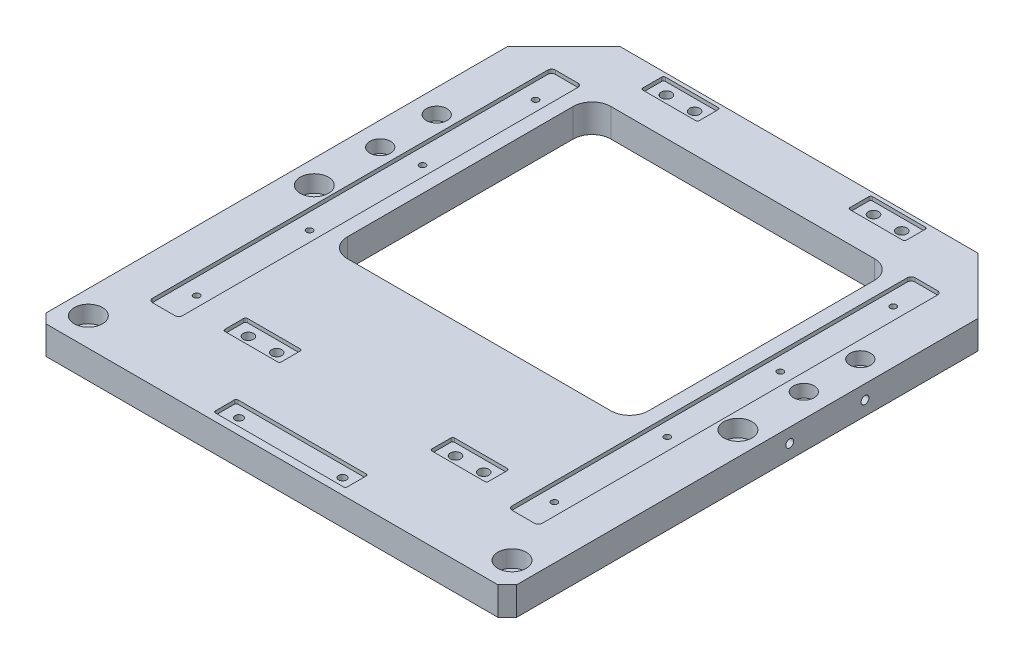
from build123d import *

# Parameters (mm, degrees)
SKETCH_1_W                   = 250
SKETCH_1_H                   = 280
EXTRUDE_1_DEPTH              = 7.5
HOLE_WIZARD_M8_2_D           = 9
HOLE_WIZARD_M8_2_CBORE_D     = 15
HOLE_WIZARD_M8_2_CBORE_DEPTH = 9
CUT_EXTRUDE_1_DEPTH          = 15
HOLE_WIZARD_M4_1_D           = 3.3
HOLE_WIZARD_M5_1_D           = 4.2
HOLE_WIZARD_M5_2_D           = 5.5
HOLE_WIZARD_M5_2_CBORE_D     = 10
HOLE_WIZARD_M5_2_CBORE_DEPTH = 5.7
CUT_EXTRUDE_2_DEPTH          = 2
HOLE_WIZARD_M6_1_D           = 6.6
HOLE_WIZARD_M6_1_DEPTH       = 15
HOLE_WIZARD_M6_1_CBORE_D     = 11
HOLE_WIZARD_M6_1_CBORE_DEPTH = 6.8
HOLE_WIZARD_M6_1_TIP         = 1.982840043
CUT_EXTRUDE_3_DEPTH          = 2
CUT_EXTRUDE_4_DEPTH          = 2
CHAMFER_1_SIZE               = 5
CHAMFER_2_SIZE               = 30
HOLE_WIZARD_M5_2_2_D         = 4.2
HOLE_WIZARD_M5_2_2_DEPTH     = 12.4
HOLE_WIZARD_M5_2_2_TIP       = 1.2618073


with BuildPart() as part:
    # 草图1 → 凸台-拉伸1 (new, symmetric)
    with BuildSketch(Plane(origin=(0, 0, 0), x_dir=(1, 0, 0), z_dir=(0, 1, 0))):
        Rectangle(SKETCH_1_W, SKETCH_1_H)
    extrude(amount=EXTRUDE_1_DEPTH, both=True)

    # M8 六角圆柱头螺钉的柱形沉头孔2 (through all)
    with Locations(Plane(origin=(0, 7.5, 0), x_dir=(1, 0, 0), z_dir=(0, 1, 0))):
        with Locations((-112.5, -125), (112.5, -125), (112.5, -5), (-112.5, -5)):
            CounterBoreHole(HOLE_WIZARD_M8_2_D / 2, HOLE_WIZARD_M8_2_CBORE_D / 2, HOLE_WIZARD_M8_2_CBORE_DEPTH)

    # 草图4 → 切除-拉伸1 (cut)
    with BuildSketch(Plane(origin=(0, 7.5, 0), x_dir=(1, 0, 0), z_dir=(0, 1, 0))):
        with BuildLine():
            Line((-70, -30), (70, -30))
            ThreePointArc((70, -30), (77.071067812, -27.071067812), (80, -20))
            Line((80, -20), (80, 100))
            ThreePointArc((80, 100), (77.071067812, 107.071067812), (70, 110))
            Line((70, 110), (-70, 110))
            ThreePointArc((-70, 110), (-77.071067812, 107.071067812), (-80, 100))
            Line((-80, 100), (-80, -20))
            ThreePointArc((-80, -20), (-77.071067812, -27.071067812), (-70, -30))
        make_face()
    extrude(amount=-CUT_EXTRUDE_1_DEPTH, mode=Mode.SUBTRACT)

    # M4 螺纹孔1 (through all)
    with Locations(Plane(origin=(0, 7.5, 0), x_dir=(1, 0, 0), z_dir=(0, 1, 0))):
        with Locations((95, 95), (-95, 95), (-95, 35), (-95, -25), (-95, -85), (95, 35), (95, -25), (95, -85)):
            Hole(HOLE_WIZARD_M4_1_D / 2)

    # M5 螺纹孔1 (through all)
    with Locations(Plane(origin=(0, 7.5, 0), x_dir=(1, 0, 0), z_dir=(0, 1, 0))):
        with Locations((27.5, -130), (-27.5, -130)):
            Hole(HOLE_WIZARD_M5_1_D / 2)

    # Hole Wizard M5 _2 (through all)
    with Locations(Plane(origin=(0, -7.5, 0), x_dir=(-1, 0, 0), z_dir=(0, -1, 0))):
        with Locations((47.5, 132), (62.5, 132), (62.5, -90), (47.5, -90), (-47.5, -90), (-62.5, -90), (-62.5, 132), (-47.5, 132)):
            CounterBoreHole(HOLE_WIZARD_M5_2_D / 2, HOLE_WIZARD_M5_2_CBORE_D / 2, HOLE_WIZARD_M5_2_CBORE_DEPTH)

    # 草图11 → 切除-拉伸2 (cut)
    with BuildSketch(Plane(origin=(0, 7.5, 0), x_dir=(1, 0, 0), z_dir=(0, 1, 0))):
        with BuildLine():
            Line((101.5, -102), (89.5, -102))
            ThreePointArc((89.5, -102), (88.085786438, -101.414213562), (87.5, -100))
            Line((87.5, -100), (87.5, 110))
            ThreePointArc((87.5, 110), (88.085786438, 111.414213562), (89.5, 112))
            Line((89.5, 112), (101.5, 112))
            ThreePointArc((101.5, 112), (102.914213562, 111.414213562), (103.5, 110))
            Line((103.5, 110), (103.5, -100))
            ThreePointArc((103.5, -100), (102.914213562, -101.414213562), (101.5, -102))
        make_face()
        with BuildLine():
            Line((-87.5, -100), (-87.5, 110))
            ThreePointArc((-87.5, 110), (-88.085786438, 111.414213562), (-89.5, 112))
            Line((-89.5, 112), (-101.5, 112))
            ThreePointArc((-101.5, 112), (-102.914213562, 111.414213562), (-103.5, 110))
            Line((-103.5, 110), (-103.5, -100))
            ThreePointArc((-103.5, -100), (-102.914213562, -101.414213562), (-101.5, -102))
            Line((-101.5, -102), (-89.5, -102))
            ThreePointArc((-89.5, -102), (-88.085786438, -101.414213562), (-87.5, -100))
        make_face()
    extrude(amount=-CUT_EXTRUDE_2_DEPTH, mode=Mode.SUBTRACT)

    # M6 六角圆柱头螺钉的柱形沉头孔1
    with Locations(Plane(origin=(0, 7.5, 0), x_dir=(1, 0, 0), z_dir=(0, 1, 0))):
        with Locations((-112.5, 30), (-112.5, 60), (112.5, 60), (112.5, 30)):
            CounterBoreHole(HOLE_WIZARD_M6_1_D / 2, HOLE_WIZARD_M6_1_CBORE_D / 2, HOLE_WIZARD_M6_1_CBORE_DEPTH, depth=HOLE_WIZARD_M6_1_DEPTH)
            with Locations((0, 0, -(HOLE_WIZARD_M6_1_DEPTH + HOLE_WIZARD_M6_1_TIP / 2))):  # 118° drill point
                Cone(0, HOLE_WIZARD_M6_1_D / 2, HOLE_WIZARD_M6_1_TIP, mode=Mode.SUBTRACT)

    # 草图14 → 切除-拉伸3 (cut)
    with BuildSketch(Plane(origin=(0, 7.5, 0), x_dir=(1, 0, 0), z_dir=(0, 1, 0))):
        with BuildLine():
            Line((-41, 138), (-69, 138))
            ThreePointArc((-69, 138), (-69.707106781, 137.707106781), (-70, 137))
            Line((-70, 137), (-70, 127))
            ThreePointArc((-70, 127), (-69.707106781, 126.292893219), (-69, 126))
            Line((-69, 126), (-41, 126))
            ThreePointArc((-41, 126), (-40.292893219, 126.292893219), (-40, 127))
            Line((-40, 127), (-40, 137))
            ThreePointArc((-40, 137), (-40.292893219, 137.707106781), (-41, 138))
        make_face()
        with BuildLine():
            Line((70, 137), (70, 127))
            ThreePointArc((70, 127), (69.707106781, 126.292893219), (69, 126))
            Line((69, 126), (41, 126))
            ThreePointArc((41, 126), (40.292893219, 126.292893219), (40, 127))
            Line((40, 127), (40, 137))
            ThreePointArc((40, 137), (40.292893219, 137.707106781), (41, 138))
            Line((41, 138), (69, 138))
            ThreePointArc((69, 138), (69.707106781, 137.707106781), (70, 137))
        make_face()
        with BuildLine():
            Line((41, -96), (69, -96))
            ThreePointArc((69, -96), (69.707106781, -95.707106781), (70, -95))
            Line((70, -95), (70, -85))
            ThreePointArc((70, -85), (69.707106781, -84.292893219), (69, -84))
            Line((69, -84), (41, -84))
            ThreePointArc((41, -84), (40.292893219, -84.292893219), (40, -85))
            Line((40, -85), (40, -95))
            ThreePointArc((40, -95), (40.292893219, -95.707106781), (41, -96))
        make_face()
        with BuildLine():
            Line((-70, -95), (-70, -85))
            ThreePointArc((-70, -85), (-69.707106781, -84.292893219), (-69, -84))
            Line((-69, -84), (-41, -84))
            ThreePointArc((-41, -84), (-40.292893219, -84.292893219), (-40, -85))
            Line((-40, -85), (-40, -95))
            ThreePointArc((-40, -95), (-40.292893219, -95.707106781), (-41, -96))
            Line((-41, -96), (-69, -96))
            ThreePointArc((-69, -96), (-69.707106781, -95.707106781), (-70, -95))
        make_face()
    extrude(amount=-CUT_EXTRUDE_3_DEPTH, mode=Mode.SUBTRACT)

    # 草图15 → 切除-拉伸4 (cut)
    with BuildSketch(Plane(origin=(0, 7.5, 0), x_dir=(1, 0, 0), z_dir=(0, 1, 0))):
        with BuildLine():
            Line((34, -124), (-34, -124))
            ThreePointArc((-34, -124), (-34.707106781, -124.292893219), (-35, -125))
            Line((-35, -125), (-35, -135))
            ThreePointArc((-35, -135), (-34.707106781, -135.707106781), (-34, -136))
            Line((-34, -136), (34, -136))
            ThreePointArc((34, -136), (34.707106781, -135.707106781), (35, -135))
            Line((35, -135), (35, -125))
            ThreePointArc((35, -125), (34.707106781, -124.292893219), (34, -124))
        make_face()
    extrude(amount=-CUT_EXTRUDE_4_DEPTH, mode=Mode.SUBTRACT)

    # 倒角1
    chamfer_1_edges = [part.edges().sort_by_distance(p)[0] for p in [
        (125, 0, 140),
        (-125, 0, 140),
    ]]
    chamfer(chamfer_1_edges, length=CHAMFER_1_SIZE)

    # 倒角2
    chamfer_2_edges = [part.edges().sort_by_distance(p)[0] for p in [
        (-125, 0, -140),
        (125, 0, -140),
    ]]
    chamfer(chamfer_2_edges, length=CHAMFER_2_SIZE)

    # Hole Wizard M5 _2 2
    with Locations(Plane(origin=(125, 0, 0), x_dir=(0, 0, -1), z_dir=(1, 0, 0))):
        with Locations((10, 0), (50, 0)):
            Hole(HOLE_WIZARD_M5_2_2_D / 2, depth=HOLE_WIZARD_M5_2_2_DEPTH)
            with Locations((0, 0, -(HOLE_WIZARD_M5_2_2_DEPTH + HOLE_WIZARD_M5_2_2_TIP / 2))):  # 118° drill point
                Cone(0, HOLE_WIZARD_M5_2_2_D / 2, HOLE_WIZARD_M5_2_2_TIP, mode=Mode.SUBTRACT)


solid = part.part
